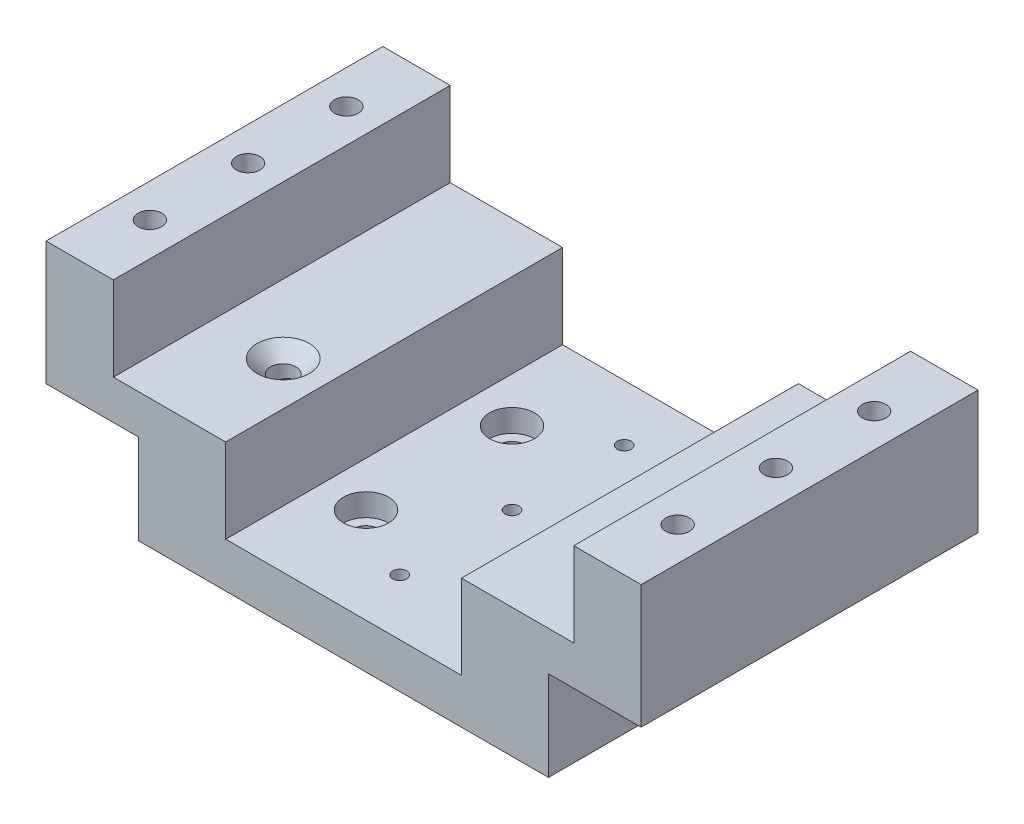
from build123d import *

# Parameters (mm, degrees)
EXTRUDE_1_DEPTH              = 30
HOLE_WIZARD_M5_1_AT_2_COUNT  = 2
HOLE_WIZARD_M5_1_AT_2_PITCH  = 35
HOLE_WIZARD_M5_1_AT_3_COUNT  = 2
HOLE_WIZARD_M5_1_AT_3_PITCH  = 17.5
SKETCH_15_W                  = 50
SKETCH_15_H                  = 47.549368588
CUT_EXTRUDE_7_DEPTH          = 89.617154096
HOLE_WIZARD_2_D              = 4.5
HOLE_WIZARD_2_CBORE_D        = 8
HOLE_WIZARD_2_CBORE_DEPTH    = 4
HOLE_WIZARD_M3_4_D           = 2.5
HOLE_WIZARD_M3_4_DEPTH       = 12.5
HOLE_WIZARD_M3_4_TIP         = 0.751075774
HOLE_WIZARD_M3_5_D           = 2.5
PATTERN_LINEAR_1_COUNT       = 3
PATTERN_LINEAR_1_PITCH       = 20
HOLE_WIZARD_M3_6_D           = 2.5
HOLE_WIZARD_M3_6_DEPTH       = 8.5
HOLE_WIZARD_M3_6_TIP         = 0.751075774
MOVE_FACE_1_BY               = 4
MOVE_FACE_1_2_BY             = 4
SKETCH_37_R                  = 5.5
CUT_EXTRUDE_10_DEPTH         = 50
CHAMFER_2_SIZE               = 1
HOLE_WIZARD_1_D              = 4.5
HOLE_WIZARD_1_DEPTH          = 11.5
HOLE_WIZARD_1_CSINK_D        = 9.3
HOLE_WIZARD_1_CSINK_ANGLE    = 90
HOLE_WIZARD_1_TIP            = 1.351936393
SKETCH_38_R                  = 0.707693856
CUT_EXTRUDE_11_DEPTH         = 33
HOLE_WIZARD_M4_1_D           = 3.3
HOLE_WIZARD_M4_1_DEPTH       = 10.1
HOLE_WIZARD_M4_1_CSINK_D     = 4.05
HOLE_WIZARD_M4_1_CSINK_ANGLE = 90
HOLE_WIZARD_M4_1_TIP         = 0.991420021


with BuildPart() as part:
    # 草图1 → 凸台-拉伸1 (new, symmetric)
    with BuildSketch(Plane.XY):
        Polygon((36.5, 0), (-36.5, 0), (-36.5, 16), (-53, 16), (-53, 38), (-41, 38), (-41, 23), (-21, 23), (-21, 8), (21, 8), (21, 23), (41, 23), (41, 38), (53, 38), (53, 16), (36.5, 16), align=None)
    extrude(amount=EXTRUDE_1_DEPTH, both=True)

    # 草图9 → M5 螺纹孔1 (revolve, cut)
    with BuildSketch(Plane(origin=(-47, 38, -17.5), x_dir=(0, 0, 1), z_dir=(1, 0, 0))):
        Polygon((0, 0), (0, 15.6618073), (2.1, 14.4), (2.1, 0), align=None)
    hole_wizard_m5_1 = revolve(axis=Axis((-47, 44.35, -17.5), (0, -1, 0)), mode=Mode.SUBTRACT)

    # M5 螺纹孔1 at 2: M5 螺纹孔1 ×2
    with Locations(*[(0, 0, i * HOLE_WIZARD_M5_1_AT_2_PITCH) for i in range(1, HOLE_WIZARD_M5_1_AT_2_COUNT)]):
        add(hole_wizard_m5_1, mode=Mode.SUBTRACT)

    # M5 螺纹孔1 at 3: M5 螺纹孔1 ×2
    with Locations(*[(0, 0, i * HOLE_WIZARD_M5_1_AT_3_PITCH) for i in range(1, HOLE_WIZARD_M5_1_AT_3_COUNT)]):
        add(hole_wizard_m5_1, mode=Mode.SUBTRACT)

    # 镜向1: M5 螺纹孔1 across plane
    add(hole_wizard_m5_1.mirror(Plane(origin=(0, 0, 0), x_dir=(0, 0, 1), z_dir=(1, 0, 0))), mode=Mode.SUBTRACT)

    # 镜向1 copy 1 sketch → 镜向1 copy 1 (revolve, cut)
    with BuildSketch(Plane(origin=(47, 38, 17.5), x_dir=(0, 0, 1), z_dir=(-1, 0, 0))):
        Polygon((0, 0), (0, -15.6618073), (2.1, -14.4), (2.1, 0), align=None)
    revolve(axis=Axis((47, 44.35, 17.5), (0, 1, 0)), mode=Mode.SUBTRACT)

    # 镜向1 copy 2 sketch → 镜向1 copy 2 (revolve, cut)
    with BuildSketch(Plane(origin=(47, 38, 0), x_dir=(0, 0, 1), z_dir=(-1, 0, 0))):
        Polygon((0, 0), (0, -15.6618073), (2.1, -14.4), (2.1, 0), align=None)
    revolve(axis=Axis((47, 44.35, 0), (0, 1, 0)), mode=Mode.SUBTRACT)

    # 草图15 → 切除-拉伸7 (cut, through all)
    with BuildSketch(Plane.XY.offset(30)):
        with Locations((0, 31.774684294)):
            Rectangle(SKETCH_15_W, SKETCH_15_H)
    extrude(amount=-CUT_EXTRUDE_7_DEPTH, mode=Mode.SUBTRACT)

    # 打孔尺寸(%根据)开槽圆柱头螺钉的类型2 (through all)
    with Locations(Plane(origin=(0, 8, 0), x_dir=(1, 0, 0), z_dir=(0, 1, 0))):
        with Locations((-13, 13), (13, 13), (-13, -13), (13, -13)):
            CounterBoreHole(HOLE_WIZARD_2_D / 2, HOLE_WIZARD_2_CBORE_D / 2, HOLE_WIZARD_2_CBORE_DEPTH)

    # M3 螺纹孔4
    with Locations(Plane(origin=(0, 0, -30), x_dir=(-1, 0, 0), z_dir=(0, 0, -1))):
        with Locations((8, 4), (-7, 4)):
            Hole(HOLE_WIZARD_M3_4_D / 2, depth=HOLE_WIZARD_M3_4_DEPTH)
            with Locations((0, 0, -(HOLE_WIZARD_M3_4_DEPTH + HOLE_WIZARD_M3_4_TIP / 2))):  # 118° drill point
                Cone(0, HOLE_WIZARD_M3_4_D / 2, HOLE_WIZARD_M3_4_TIP, mode=Mode.SUBTRACT)

    # M3 螺纹孔5 (through all)
    with Locations(Plane(origin=(0, 8, 20), x_dir=(0, 0, 1), z_dir=(0, 1, 0))):
        with Locations((0, 0)):
            hole_wizard_m3_5 = Hole(HOLE_WIZARD_M3_5_D / 2)

    # 阵列(线性)1: M3 螺纹孔5 ×3
    with Locations(*[(0, 0, -i * PATTERN_LINEAR_1_PITCH) for i in range(1, PATTERN_LINEAR_1_COUNT)]):
        add(hole_wizard_m3_5, mode=Mode.SUBTRACT)

    # M3 螺纹孔6
    with Locations(Plane(origin=(33, 18, -30), x_dir=(-1, 0, 0), z_dir=(0, 0, -1))):
        with Locations((0, 0), (0, -6)):
            Hole(HOLE_WIZARD_M3_6_D / 2, depth=HOLE_WIZARD_M3_6_DEPTH)
            with Locations((0, 0, -(HOLE_WIZARD_M3_6_DEPTH + HOLE_WIZARD_M3_6_TIP / 2))):  # 118° drill point
                Cone(0, HOLE_WIZARD_M3_6_D / 2, HOLE_WIZARD_M3_6_TIP, mode=Mode.SUBTRACT)

    # Move Face 1: a face moved outward by 4.0
    extrude(part.faces().sort_by_distance((-25, 15.5, 0))[0], amount=MOVE_FACE_1_BY, dir=(1, 0, 0))

    # Move Face 1 2: a face moved outward by 4.0
    extrude(part.faces().sort_by_distance((25, 15.5, 0))[0], amount=MOVE_FACE_1_2_BY, dir=(-1, 0, 0))

    # 草图37 → 切除-拉伸10 (cut)
    with BuildSketch(Plane(origin=(0, 0, -30), x_dir=(-1, 0, 0), z_dir=(0, 0, -1))):
        with Locations((28.75, 13)):
            Circle(SKETCH_37_R)
    extrude(amount=-CUT_EXTRUDE_10_DEPTH, mode=Mode.SUBTRACT)

    # 倒角2
    chamfer_2_edges = [part.edges().sort_by_distance(p)[0] for p in [
        (-23.25, 13, -30),
    ]]
    chamfer(chamfer_2_edges, length=CHAMFER_2_SIZE)

    # 打孔尺寸(%根据)内六角花形半沉头螺钉的类型1
    with Locations(Plane(origin=(-28.75, 23, 12), x_dir=(0, 0, 1), z_dir=(0, 1, 0))):
        with Locations((0, 0)):
            CounterSinkHole(HOLE_WIZARD_1_D / 2, HOLE_WIZARD_1_CSINK_D / 2, depth=HOLE_WIZARD_1_DEPTH, counter_sink_angle=HOLE_WIZARD_1_CSINK_ANGLE)
            with Locations((0, 0, -(HOLE_WIZARD_1_DEPTH + HOLE_WIZARD_1_TIP / 2))):  # 118° drill point
                Cone(0, HOLE_WIZARD_1_D / 2, HOLE_WIZARD_1_TIP, mode=Mode.SUBTRACT)

    # 草图38 → 切除-拉伸11 (cut)
    with BuildSketch(Plane(origin=(0, 23, 0), x_dir=(1, 0, 0), z_dir=(0, 1, 0))):
        with Locations(Location((-28.75, -12, 0), (0, 0, 270))):
            Circle(SKETCH_38_R)
    extrude(amount=-CUT_EXTRUDE_11_DEPTH, mode=Mode.SUBTRACT)

    # M4 螺纹孔1
    with Locations(Plane(origin=(-28.75, 0, 12), x_dir=(0, 0, -1), z_dir=(0, -1, 0))):
        with Locations((0, 0)):
            CounterSinkHole(HOLE_WIZARD_M4_1_D / 2, HOLE_WIZARD_M4_1_CSINK_D / 2, depth=HOLE_WIZARD_M4_1_DEPTH, counter_sink_angle=HOLE_WIZARD_M4_1_CSINK_ANGLE)
            with Locations((0, 0, -(HOLE_WIZARD_M4_1_DEPTH + HOLE_WIZARD_M4_1_TIP / 2))):  # 118° drill point
                Cone(0, HOLE_WIZARD_M4_1_D / 2, HOLE_WIZARD_M4_1_TIP, mode=Mode.SUBTRACT)


solid = part.part
